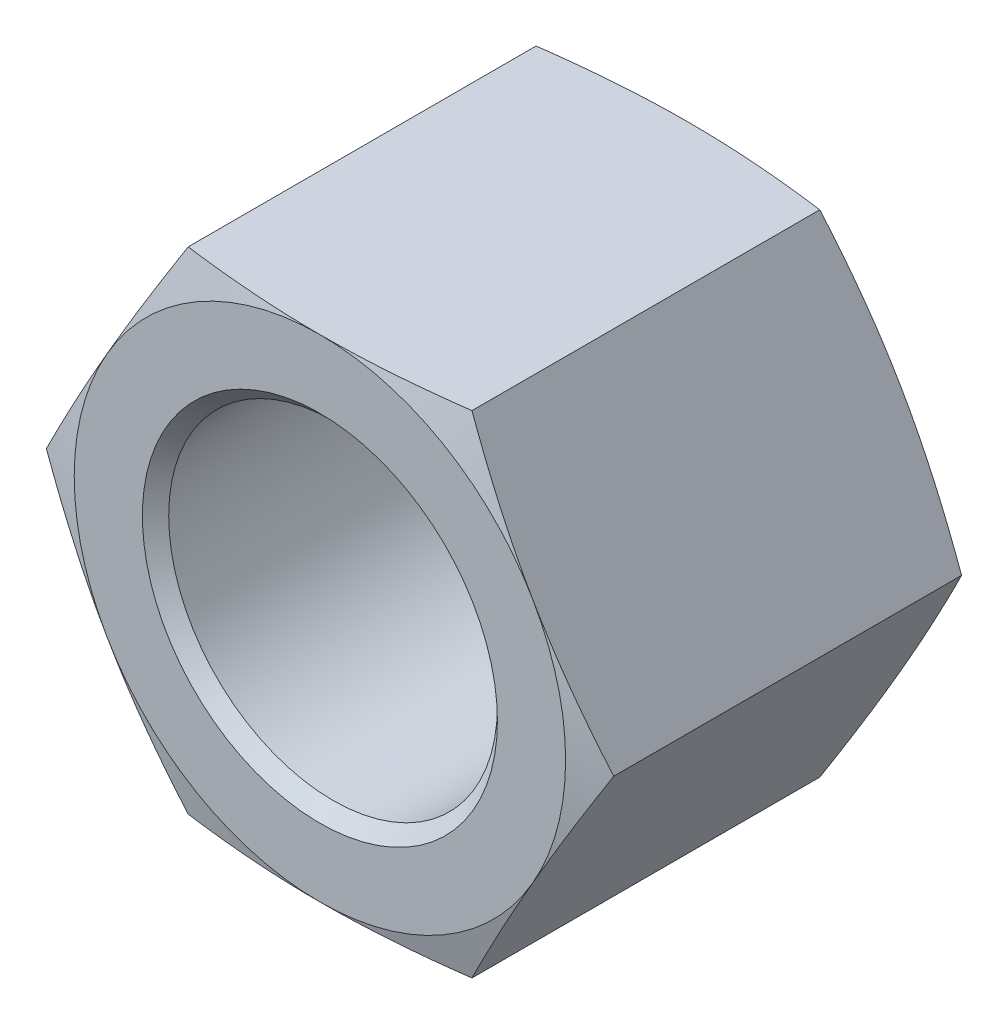
from build123d import *

# Parameters (mm, degrees)
SKETCH1_R          = 2.5
BOSS_EXTRUDE_DEPTH = 5.6
SKETCH2_OUTSIDE_W  = 296.81
SKETCH2_OUTSIDE_H  = 295.654
SKETCH2_OUTSIDE_R  = 3.736899617
CUT_EXTRUDE1_DEPTH = 38
CUT_EXTRUDE1_DRAFT = -75
SKETCH3_OUTSIDE_W  = 296.81
SKETCH3_OUTSIDE_H  = 295.654
SKETCH3_OUTSIDE_R  = 3.736899617
CUT_EXTRUDE2_DEPTH = 38
CUT_EXTRUDE2_DRAFT = -75
CHAMFER1_SIZE      = 0.2


with BuildPart() as part:
    # Sketch1 → Boss-Extrude (new body)
    with BuildSketch(Plane.XY):
        Polygon((2.1575, 3.736899617), (-2.1575, 3.736899617), (-4.315, 0), (-2.1575, -3.736899617), (2.1575, -3.736899617), (4.315, 0), align=None)
        Circle(SKETCH1_R, mode=Mode.SUBTRACT)
    extrude(amount=BOSS_EXTRUDE_DEPTH)


with BuildPart() as cut_extrude1_tool:
    # Sketch2 outside → Cut-Extrude1 (with draft: the straight prism first)
    with BuildSketch(Plane(origin=(0, 0, 0), x_dir=(-1, 0, 0), z_dir=(0, 0, -1))):
        Rectangle(SKETCH2_OUTSIDE_W, SKETCH2_OUTSIDE_H)
        Circle(SKETCH2_OUTSIDE_R, mode=Mode.SUBTRACT)
    extrude(amount=-CUT_EXTRUDE1_DEPTH)
    # Cut-Extrude1: the draft: its side faces are tilted about the plane it starts from
    cut_extrude1_sides = [cut_extrude1_tool.faces().sort_by_distance(p)[0] for p in [
        (0, -147.827, 19),
        (-148.405, 0, 19),
        (0, 147.827, 19),
        (148.405, 0, 19),
        (3.736899617, 0, 19),
    ]]
    draft(cut_extrude1_sides, Plane(origin=(0, 0, 0), x_dir=(-1, 0, 0), z_dir=(0, 0, -1)), CUT_EXTRUDE1_DRAFT)


with BuildPart() as part_1:
    add(part.part)

    # Cut-Extrude1: cut by cut_extrude1_tool
    add(cut_extrude1_tool.part, mode=Mode.SUBTRACT)


with BuildPart() as cut_extrude2_tool:
    # Sketch3 outside → Cut-Extrude2 (with draft: the straight prism first)
    with BuildSketch(Plane.XY.offset(5.6)):
        Rectangle(SKETCH3_OUTSIDE_W, SKETCH3_OUTSIDE_H)
        Circle(SKETCH3_OUTSIDE_R, mode=Mode.SUBTRACT)
    extrude(amount=-CUT_EXTRUDE2_DEPTH)
    # Cut-Extrude2: the draft: its side faces are tilted about the plane it starts from
    cut_extrude2_sides = [cut_extrude2_tool.faces().sort_by_distance(p)[0] for p in [
        (0, -147.827, -13.4),
        (148.405, 0, -13.4),
        (0, 147.827, -13.4),
        (-148.405, 0, -13.4),
        (-3.736899617, 0, -13.4),
    ]]
    draft(cut_extrude2_sides, Plane.XY.offset(5.6), CUT_EXTRUDE2_DRAFT)


with BuildPart() as part_2:
    add(part_1.part)

    # Cut-Extrude2: cut by cut_extrude2_tool
    add(cut_extrude2_tool.part, mode=Mode.SUBTRACT)

    # Chamfer1
    chamfer1_edges = [part_2.edges().sort_by_distance(p)[0] for p in [
        (-2.5, 0, 0),
        (-2.5, 0, 5.6),
    ]]
    chamfer(chamfer1_edges, length=CHAMFER1_SIZE)


solid = part_2.part
